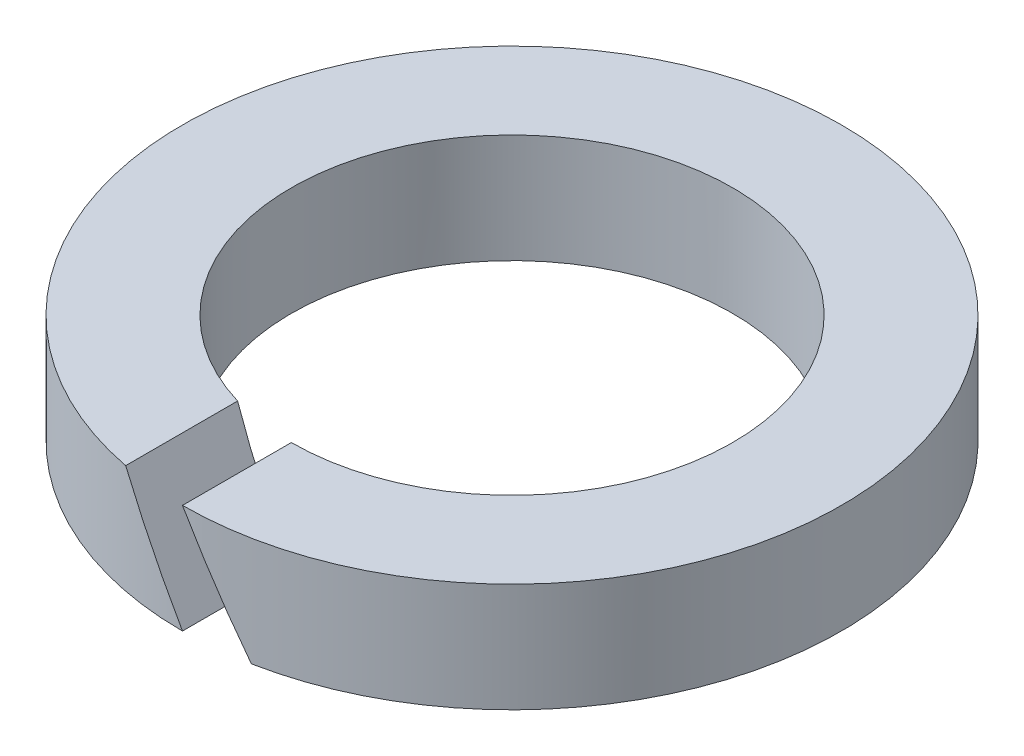
SolidWorks part; units mm, degrees
material "65Mn"
ref_plane "Front Plane" through (0, 0, 0) normal (0, 0, 1) x (1, 0, 0)
ref_plane "Top Plane" through (0, 0, 0) normal (0, 1, 0) x (1, 0, 0)
ref_plane "Right Plane" through (0, 0, 0) normal (1, 0, 0) x (0, 0, -1)
sketch "Sketch1" plane through (0, 0, 0) normal (0, 1, 0) x (1, 0, 0)
  circle A0 centre (0, 0) radius 18.25
  circle A1 centre (0, 0) radius 27.25
  dimension "D1" = 54.5
  dimension "D2" = 36.5
extrude "Boss-Extrude1" add sketch "Sketch1" along normal mid plane 9
sketch "Sketch2" plane through (0, 0, 0) normal (0, 0, 1) x (1, 0, 0)
  line L0 (18.25, 4.5) -> (-18.25, 4.5) construction
  line L1 (-27.25, -4.5) -> (27.25, -4.5) construction
  line L2 (0, 4.5) -> (-5.1962, 4.5)
  line L3 (0, -4.5) -> (5.1962, -4.5)
  line L4 (-5.1962, 4.5) -> (0, -4.5)
  line L5 (0, 4.5) -> (5.1962, -4.5)
  line L6 (0, 6.5555) -> (0, -5.0854) construction
  dimension "D1" = 30
  dimension "D2" = 4.5
extrude "Cut-Extrude1" cut sketch "Sketch2" along normal through all
